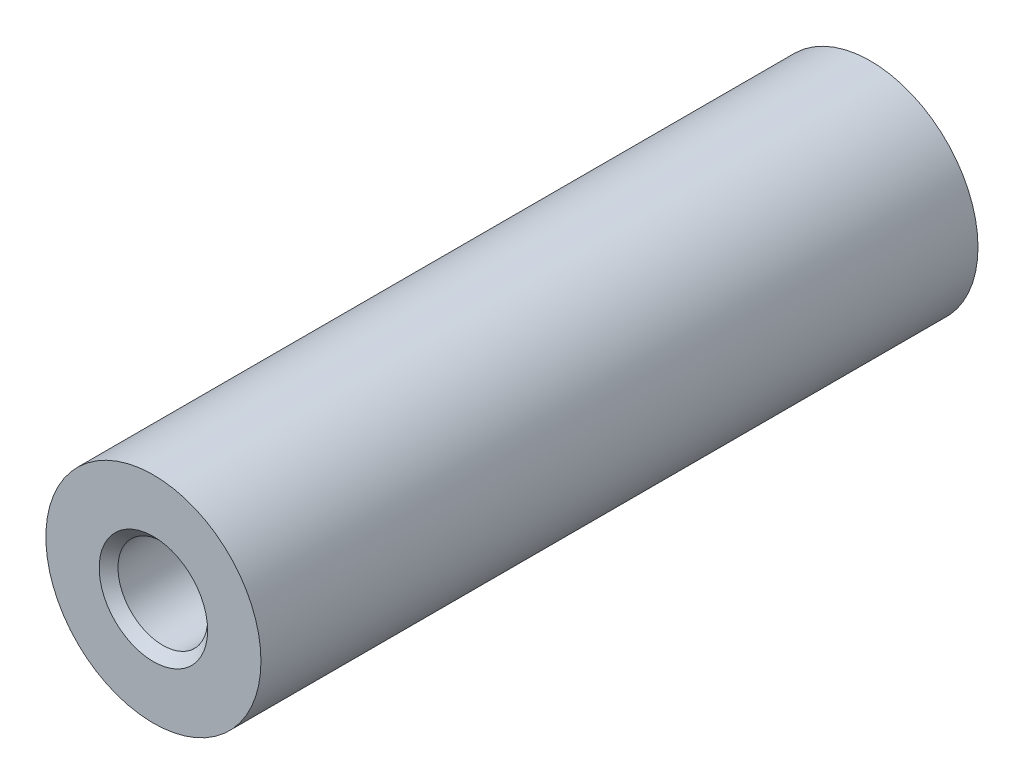
from build123d import *

# Parameters (mm, degrees)
SKETCH_1_R      = 6
EXTRUDE_1_DEPTH = 20


with BuildPart() as part:
    # 草图1 → 凸台-拉伸1 (new, symmetric)
    with BuildSketch(Plane.XY):
        Circle(SKETCH_1_R)
    extrude(amount=EXTRUDE_1_DEPTH, both=True)

    # 草图3 → M6 螺纹孔1 (revolve, cut)
    with BuildSketch(Plane(origin=(0, 0, 20), x_dir=(0, -1, 0), z_dir=(1, 0, 0))):
        Polygon((0, 0), (0, 10.502151548), (2.5, 9), (2.5, 0.525), (3.025, 0), align=None)
    hole_wizard_m6_1 = revolve(axis=Axis((0, 0, 26.35), (0, 0, -1)), mode=Mode.SUBTRACT)

    # 镜向1: M6 螺纹孔1 across plane
    add(hole_wizard_m6_1.mirror(Plane.XY), mode=Mode.SUBTRACT)


solid = part.part
